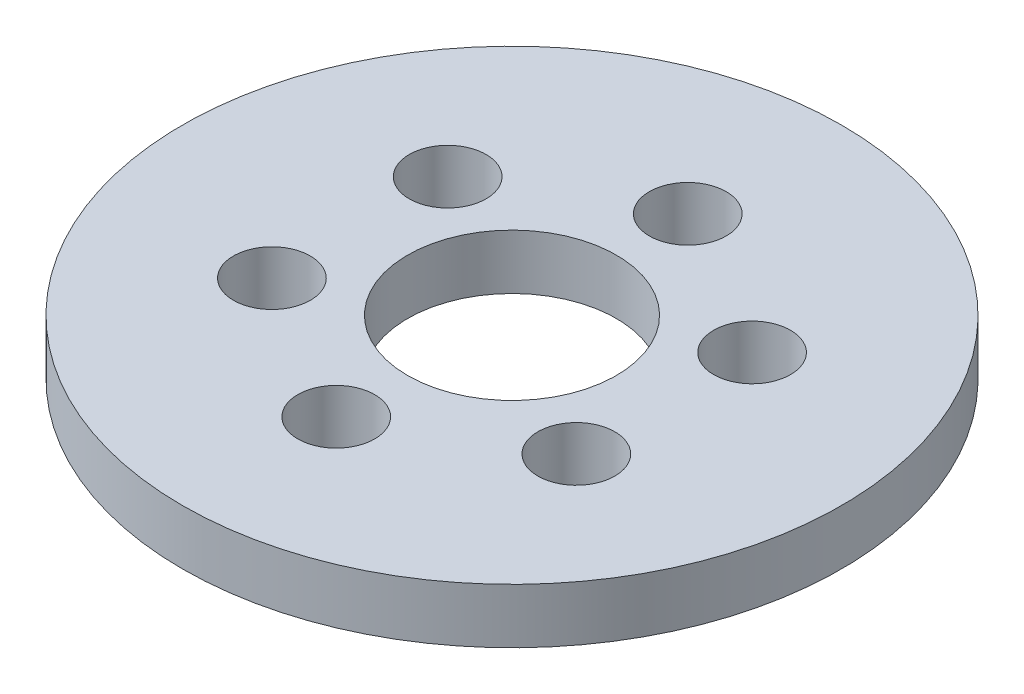
SolidWorks part; units mm, degrees
material "Q235A"
ref_plane "前视基准面" through (0, 0, 0) normal (0, 0, 1) x (1, 0, 0)
ref_plane "上视基准面" through (0, 0, 0) normal (0, 1, 0) x (1, 0, 0)
ref_plane "右视基准面" through (0, 0, 0) normal (1, 0, 0) x (0, 0, -1)
sketch "草图1" plane through (0, 0, 0) normal (0, 1, 0) x (1, 0, 0)
  circle A0 centre (0, 0) radius 9.5
  circle A1 centre (0, 0) radius 30
  dimension "D1" = 19
  dimension "D2" = 60
extrude "凸台-拉伸1" add sketch "草图1" along normal blind 5
hole_wizard "M6 间隙孔1" positions "草图2" profile "草图3" hole size "M6" standard "ISO" end condition through all
sketch "草图2" plane through (0, 5, 0) normal (0, 1, 0) x (1, 0, 0)
  line L0 (0, 0) -> (0, 16) construction
  point P0 (0, 16)
  point P9 (13.8564, 8)
  point P10 (13.8564, -8)
  point P11 (0, -16)
  point P12 (-13.8564, -8)
  point P13 (-13.8564, 8)
  dimension "D2" = 16
  dimension "D1" = 6
sketch "草图3" plane through (0, 5, -16) normal (1, 0, 0) x (0, 0, 1)
  line L0 (0, 0) -> (0, 5)
  line L1 (0, 5) -> (3.5, 5)
  line L2 (3.5, 5) -> (3.5, 0)
  line L5 (3.5, 0) -> (0, 0)
  line L11 (0, -6.35) -> (0, 107.95) construction
  dimension "通孔孔直径" = 7
  dimension "通孔孔深度" = 5
